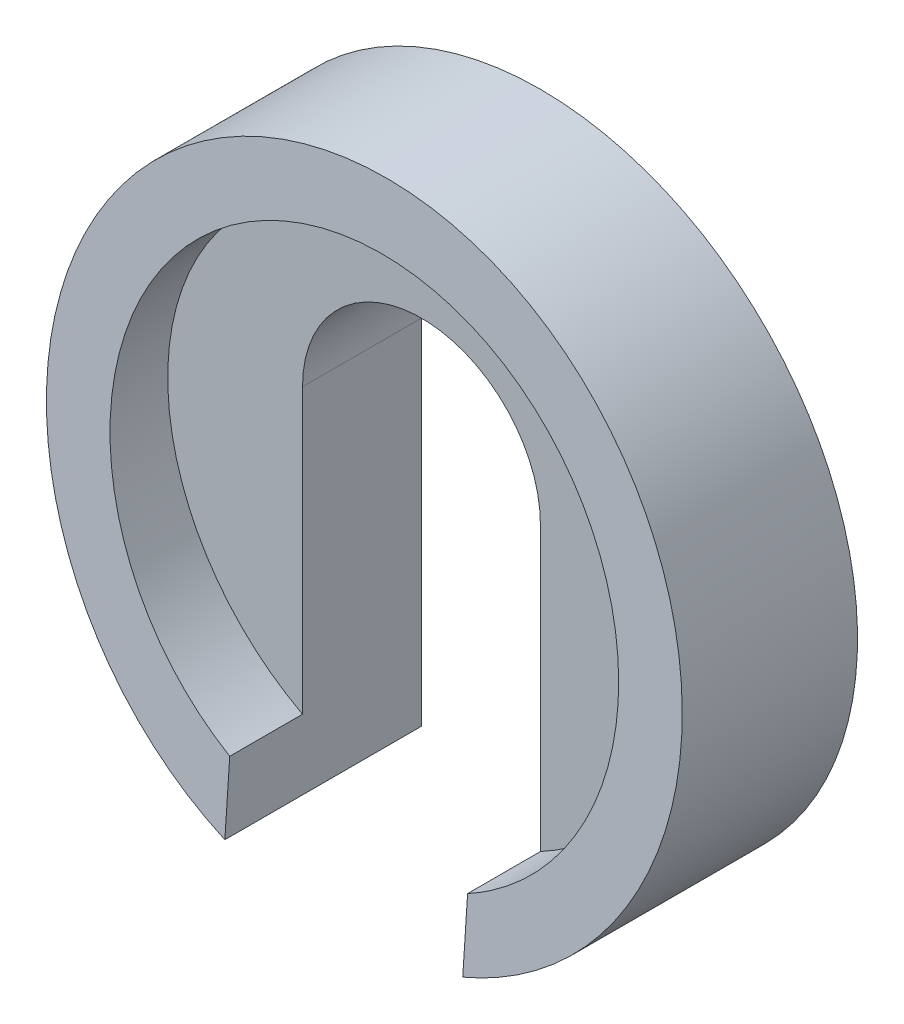
SolidWorks part; units mm, degrees
material "Q235-A"
ref_plane "Front Plane" through (0, 0, 0) normal (0, 0, 1) x (1, 0, 0)
ref_plane "Top Plane" through (0, 0, 0) normal (0, 1, 0) x (1, 0, 0)
ref_plane "Right Plane" through (0, 0, 0) normal (1, 0, 0) x (0, 0, -1)
sketch "Sketch1" plane through (0, 0, 0) normal (1, 0, 0) x (0, 0, -1)
  line L0 (85.977, 0) -> (-85.977, 0) construction
  line L2 (-50, 64) -> (-50, 80)
  line L3 (-50, 80) -> (0, 80)
  line L4 (0, 80) -> (0, 0)
  line L5 (-50, 64) -> (-30, 64)
  line L6 (-30, 64) -> (-30, 0)
  line L7 (0, 0) -> (-30, 0)
  point P4 (0, 0)
  point P6 (0, 0)
  dimension "D2" = 80
  dimension "D3" = 64
  dimension "D4" = 20
  dimension "D5" = 50
revolve "Revolve2" add sketch "Sketch1" angle 360 about L0
sketch "Sketch2" plane through (0, 0, 0) normal (1, 0, 0) x (0, 0, -1)
  line L4 (-50, 80) -> (-38.8117, 80)
  line L5 (0, 80) -> (-50, 80) construction
  line L6 (-38.8117, 80) -> (-50, -80)
  line L7 (-50, 80) -> (-50, -80) construction
  line L8 (-50, -80) -> (-50, 80)
  dimension "D2" = 4
extrude "Cut-Extrude1" cut sketch "Sketch2" against normal through all both and the other way through all
sketch "Sketch3" plane through (0, 0, 0) normal (0, 0, 1) x (1, 0, 0)
  line L0 (0, -38.523) -> (0, 38.523) construction
  line L1 (0, 15) -> (0, -100) construction
  line L2 (30, 15) -> (30, -100)
  line L3 (-30, 15) -> (-30, -100)
  arc A0 (30, 15) -> (-30, 15) centre (0, 15) ccw
  arc A1 (-30, -100) -> (30, -100) centre (0, -100) ccw
  point P4 (0, 0)
  point P6 (0, -42.5)
  dimension "D1" = 15
  dimension "D2" = 30
  dimension "D3" = 100
extrude "Cut-Extrude2" cut sketch "Sketch3" along normal through all
